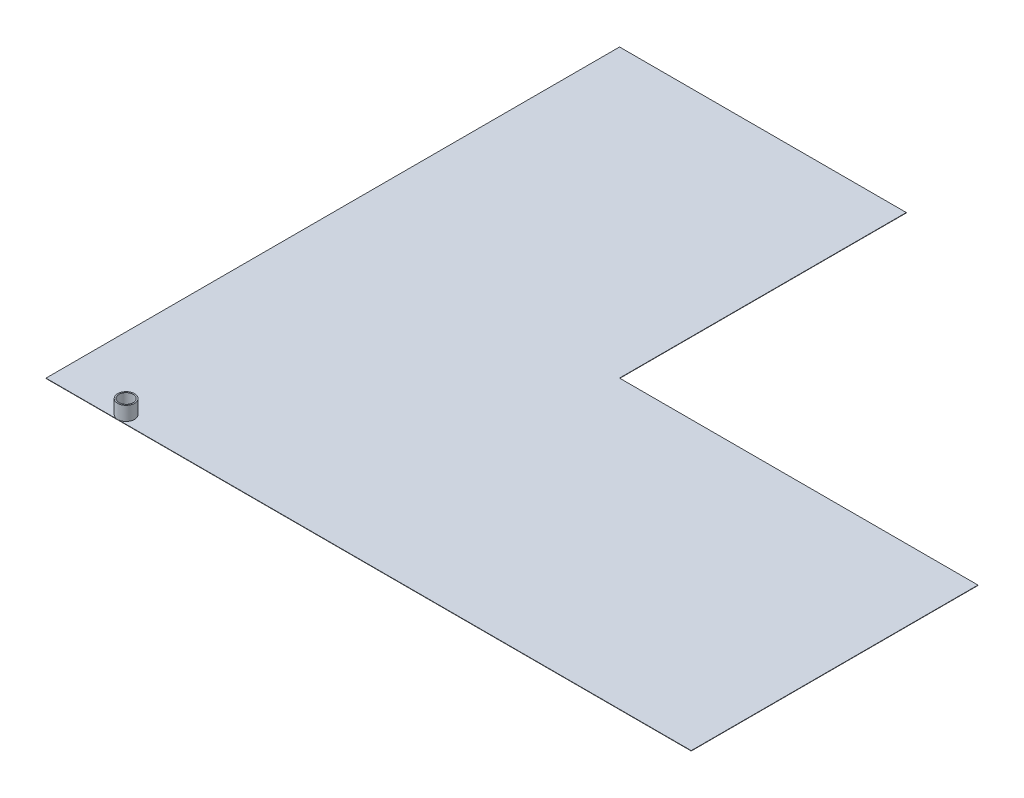
SolidWorks part; units mm, degrees
ref_plane "Front Plane" through (0, 0, 0) normal (0, 0, 1) x (1, 0, 0)
ref_plane "Top Plane" through (0, 0, 0) normal (0, 1, 0) x (1, 0, 0)
ref_plane "Right Plane" through (0, 0, 0) normal (1, 0, 0) x (0, 0, -1)
sketch "Sketch1" plane through (0, 0, 0) normal (0, 1, 0) x (1, 0, 0)
  line L1 (-900, -800) -> (900, -800)
  line L2 (-900, -800) -> (-900, 800)
  line L3 (-900, 800) -> (-100, 800)
  line L4 (900, -800) -> (900, 0)
  line L5 (-900, -800) -> (0, 0) construction
  line L6 (-900, 800) -> (900, -800) construction
  line L7 (0, 0) -> (900, 0)
  line L8 (-100, 800) -> (-100, 0)
  line L9 (-100, 0) -> (0, 0)
  point P0 (0, 0)
  dimension "D1" = 1800
  dimension "D2" = 1600
extrude "Boss-Extrude1" add sketch "Sketch1" along normal blind 1
sketch "Sketch2" plane through (0, 1, 0) normal (0, 1, 0) x (1, 0, 0)
  line L0 (-900, -800) -> (900, -800) construction
  line L1 (-900, 800) -> (-900, -800) construction
  circle A0 centre (-700, -776.5) radius 20
  dimension "D1" = 40
  dimension "D2" = 23.5
  dimension "D3" = 200
extrude "Cut-Extrude1" cut sketch "Sketch2" against normal through all
sketch "Sketch3" plane through (0, 1, 0) normal (0, 1, 0) x (1, 0, 0)
  circle A0 centre (-700, -776.5) radius 23.5
  circle A1 centre (-700, -776.5) radius 20
  dimension "D1" = 47
extrude "Boss-Extrude2" add sketch "Sketch3" along normal blind 39
